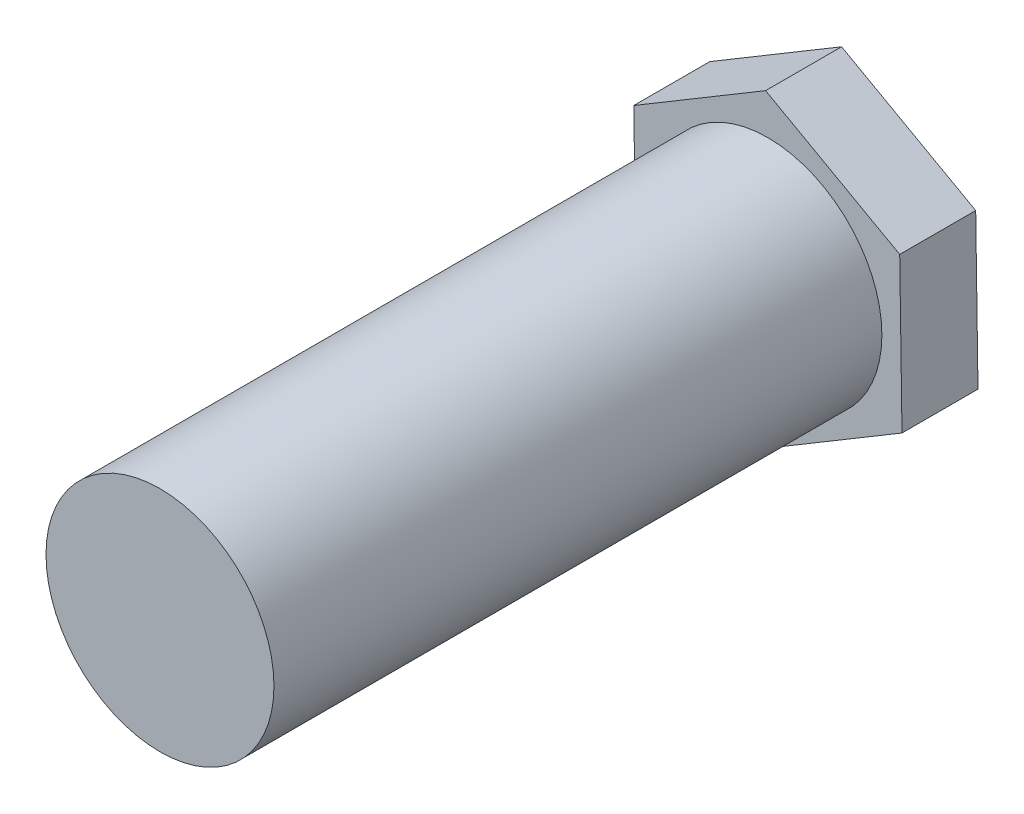
from build123d import *

# Parameters (mm, degrees)
BOSS_EXTRUDE1_DEPTH = 10
SKETCH2_R           = 15
BOSS_EXTRUDE2_DEPTH = 80


with BuildPart() as part:
    # Sketch1 → Boss-Extrude1 (new body)
    with BuildSketch(Plane.XY):
        Polygon((17.346513547, 10.364931312), (-0.303037051, 20.204987055), (-17.649550598, 9.840055742), (-17.346513547, -10.364931312), (0.303037051, -20.204987055), (17.649550598, -9.840055742), align=None)
    extrude(amount=BOSS_EXTRUDE1_DEPTH)

    # Sketch2 → Boss-Extrude2 (add)
    with BuildSketch(Plane.XY.offset(10)):
        Circle(SKETCH2_R)
    extrude(amount=BOSS_EXTRUDE2_DEPTH)


solid = part.part
